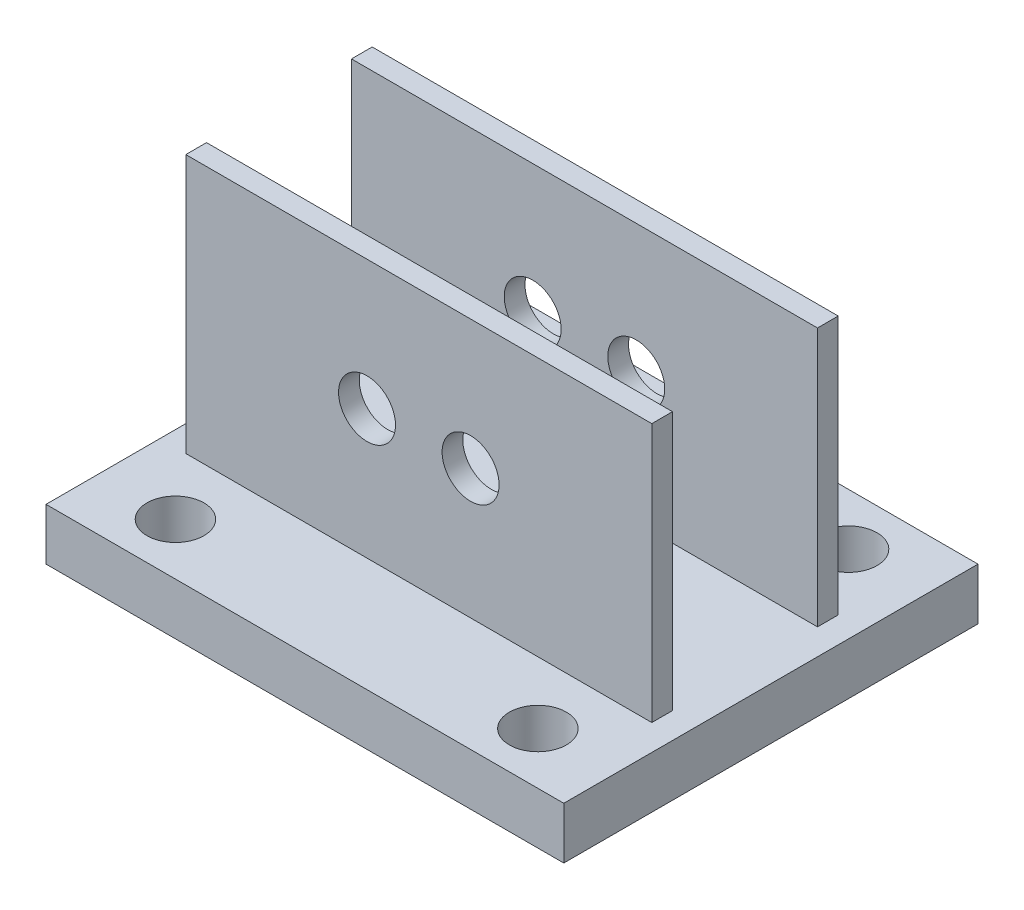
from build123d import *

# Parameters (mm, degrees)
SKETCH_1_W          = 90
SKETCH_1_H          = 50
EXTRUDE_1_DEPTH     = 4
SKETCH_2_R          = 5.5
CUT_EXTRUDE_1_DEPTH = 52.633322574
SKETCH_3_W          = 100
SKETCH_3_H          = 80
SKETCH_3_R          = 5.5
EXTRUDE_2_DEPTH     = 10
SKETCH_4_R          = 5.5
CUT_EXTRUDE_2_DEPTH = 82.492330928


with BuildPart() as part:
    # 草图1 → 凸台-拉伸1 (new body)
    with BuildSketch(Plane.XY):
        Rectangle(SKETCH_1_W, SKETCH_1_H)
    extrude_1 = extrude(amount=EXTRUDE_1_DEPTH)

    # 草图2 → 切除-拉伸1 (cut, through all)
    with BuildSketch(Plane.XY.offset(4)):
        with Locations((-10, 0)):
            Circle(SKETCH_2_R)
        with Locations((10, 0)):
            Circle(SKETCH_2_R)
    extrude(amount=-CUT_EXTRUDE_1_DEPTH, mode=Mode.SUBTRACT)

    # 草图3 → 凸台-拉伸2 (add)
    with BuildSketch(Plane.XZ.offset(25)):
        with Locations((0, -14)):
            Rectangle(SKETCH_3_W, SKETCH_3_H)
        with Locations(Location((-35, 16, 0), (0, 0, 270))):
            Circle(SKETCH_3_R, mode=Mode.SUBTRACT)
        with Locations(Location((35, 16, 0), (0, 0, 270))):
            Circle(SKETCH_3_R, mode=Mode.SUBTRACT)
        with Locations(Location((35, -44, 0), (0, 0, 270))):
            Circle(SKETCH_3_R, mode=Mode.SUBTRACT)
        with Locations(Location((-35, -44, 0), (0, 0, 270))):
            Circle(SKETCH_3_R, mode=Mode.SUBTRACT)
    extrude(amount=EXTRUDE_2_DEPTH)

    # 镜向1: 凸台-拉伸1 across plane
    add(extrude_1.mirror(Plane(origin=(0, 0, -14), x_dir=(1, 0, 0), z_dir=(0, 0, -1))))

    # 草图4 → 切除-拉伸2 (cut, through all)
    with BuildSketch(Plane.XY.offset(-28)):
        with Locations((-10, 0)):
            Circle(SKETCH_4_R)
        with Locations((10, 0)):
            Circle(SKETCH_4_R)
    extrude(amount=-CUT_EXTRUDE_2_DEPTH, mode=Mode.SUBTRACT)


solid = part.part
